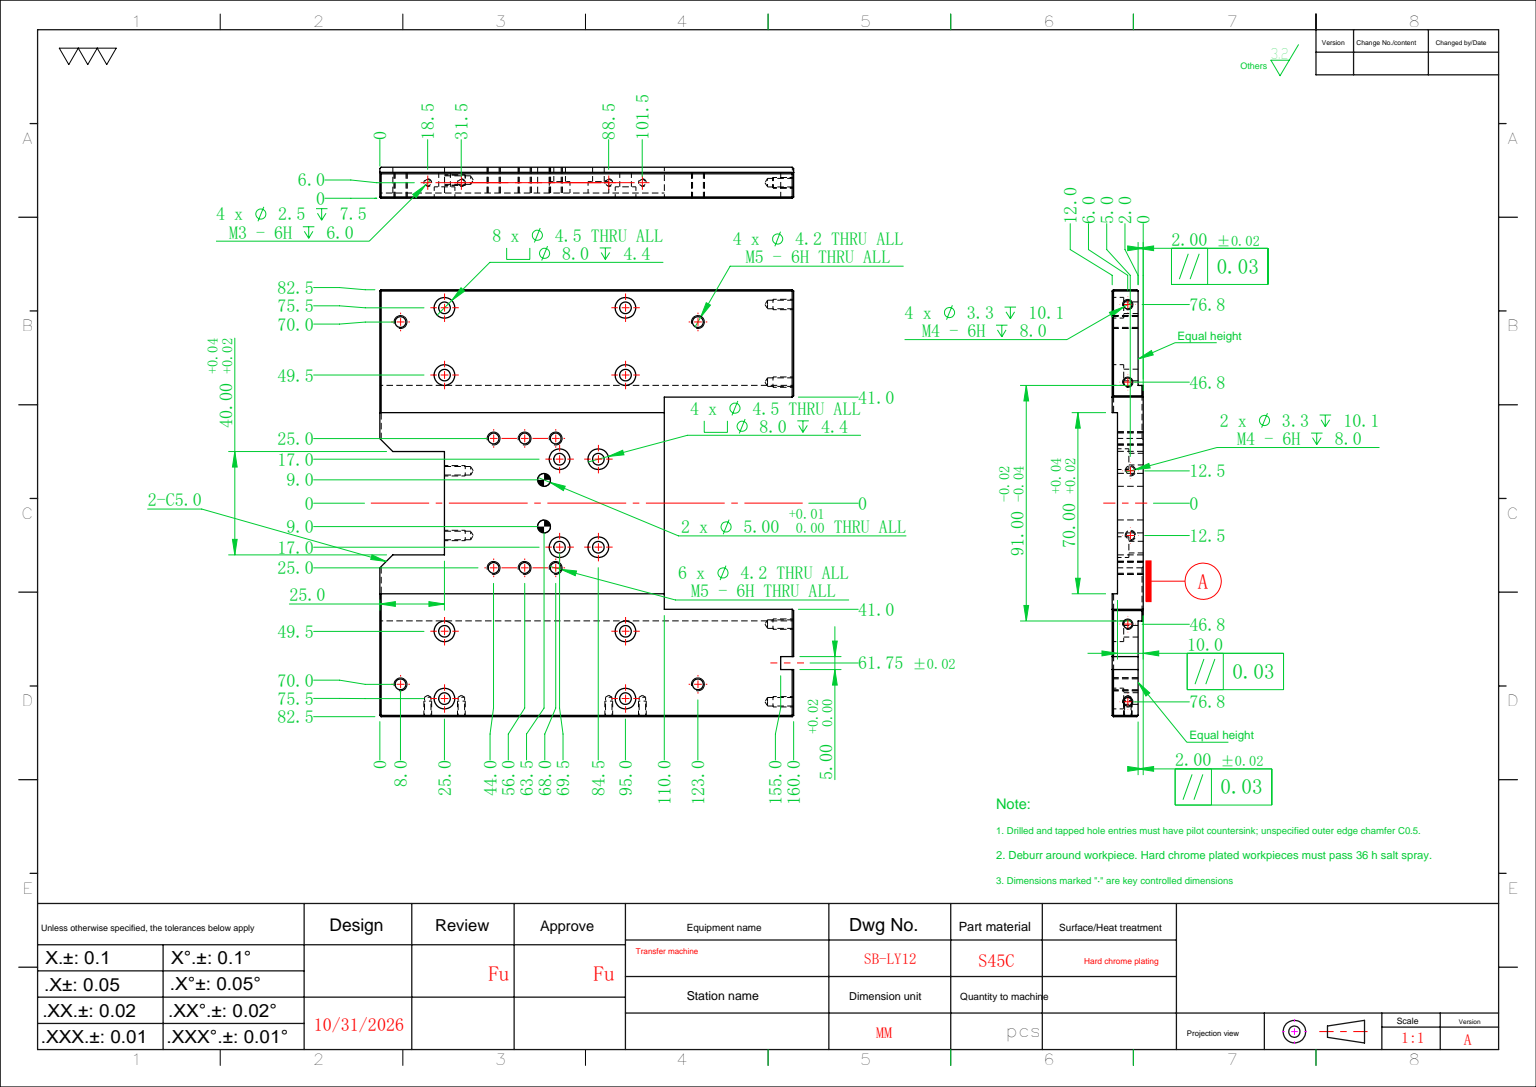
SolidWorks part; units mm, degrees
ref_plane "前视基准面" through (0, 0, 0) normal (0, 0, 1) x (1, 0, 0)
ref_plane "上视基准面" through (0, 0, 0) normal (0, 1, 0) x (1, 0, 0)
ref_plane "右视基准面" through (0, 0, 0) normal (1, 0, 0) x (0, 0, -1)
sketch "草图1" plane through (0, 0, 0) normal (0, 0, 1) x (1, 0, 0)
  line L1 (-80, -82.5) -> (80, -82.5)
  line L2 (-80, -82.5) -> (-80, 82.5)
  line L3 (-80, 82.5) -> (80, 82.5)
  line L4 (80, -82.5) -> (80, 82.5)
  line L5 (-80, -82.5) -> (80, 82.5) construction
  line L6 (-80, 82.5) -> (80, -82.5) construction
  point P0 (0, 0)
  dimension "D1" = 160
  dimension "D2" = 165
extrude "凸台-拉伸1" add sketch "草图1" along normal blind 12
sketch "草图2" plane through (0, 0, 0) normal (0, 0, -1) x (-1, 0, 0)
  line L0 (-80, -82.5) -> (-80, 82.5) construction
  line L1 (-80, -41) -> (-30, -41)
  line L2 (-80, -41) -> (-80, 41)
  line L3 (-80, 41) -> (-30, 41)
  line L4 (-30, -41) -> (-30, 41)
  line L5 (0, 0) -> (-82.6129, 0) construction
  dimension "D1" = 82
  dimension "D2" = 50
extrude "切除-拉伸1" cut sketch "草图2" against normal through all
sketch "草图3" plane through (-80, 0, 0) normal (-1, 0, 0) x (0, 0, 1)
  line L0 (12, 82.5) -> (12, -82.5) construction
  line L1 (12, 79.5) -> (10, 79.5)
  line L2 (12, 79.5) -> (12, 45.5)
  line L3 (12, 45.5) -> (10, 45.5)
  line L4 (10, 79.5) -> (10, 45.5)
  line L5 (0, 0) -> (47.3737, 0) construction
  line L6 (0, 82.5) -> (0, -82.5) construction
  line L7 (10, -79.5) -> (10, -45.5)
  line L8 (12, -45.5) -> (10, -45.5)
  line L9 (12, -79.5) -> (12, -45.5)
  line L10 (12, -79.5) -> (10, -79.5)
  line L11 (10, 62.5) -> (22.1068, 62.5) construction
  line L12 (10, -62.5) -> (25.4571, -62.5) construction
  dimension "D1" = 34
  dimension "D2" = 2
  dimension "D3" = 125
extrude "切除-拉伸2" cut sketch "草图3" against normal through all
hole_wizard "M4 六角凹头螺钉的柱形沉头孔2" positions "草图4" profile "草图5" counterbore size "M4" standard "ISO" end condition through all
sketch "草图4" plane through (0, 0, 0) normal (0, 0, -1) x (-1, 0, 0)
  line L0 (-80, 62.5) -> (-23.5435, 62.5) construction
  line L1 (-80, 79.5) -> (-80, 45.5) construction
  line L3 (0, 0) -> (127.4178, 0) construction
  line L5 (-80, -62.5) -> (-23.5435, -62.5) construction
  line L6 (-80, -45.5) -> (-80, -79.5) construction
  point P0 (-15, 49.5)
  point P2 (-15, 75.5)
  point P19 (-15, -75.5)
  point P20 (-15, -49.5)
  point P30 (55, -75.5)
  point P34 (55, -49.5)
  point P35 (55, 49.5)
  point P37 (55, 75.5)
  dimension "D1" = 26
  dimension "D3" = 65
  dimension "D5" = 70
sketch "草图5" plane through (15, 49.5, 0) normal (1, 0, 0) x (0, 1, 0)
  line L0 (0, 0) -> (0, 12)
  line L1 (0, 12) -> (2.25, 12)
  line L3 (2.25, 12) -> (2.25, 4.4)
  line L4 (2.25, 4.4) -> (4, 4.4)
  line L5 (4, 4.4) -> (4, 0)
  line L7 (4, 0) -> (0, 0)
  line L11 (0, -6.35) -> (0, 107.95) construction
  dimension "通孔孔直径" = 4.5
  dimension "通孔孔深度" = 12
  dimension "柱形沉头孔直径" = 8
  dimension "柱形沉头孔深度" = 4.4
sketch "草图6" plane through (0, 0, 0) normal (0, 0, -1) x (-1, 0, 0)
  line L0 (80, 82.5) -> (80, -82.5) construction
  line L1 (80, -35) -> (-30, -35)
  line L2 (80, -35) -> (80, 35)
  line L3 (80, 35) -> (-30, 35)
  line L4 (-30, -35) -> (-30, 35)
  line L5 (-30, -41) -> (-30, 41) construction
  line L8 (0, 0) -> (92.3084, 0) construction
  dimension "D1" = 70
extrude "切除-拉伸3" cut sketch "草图6" against normal blind 2
hole_wizard "M4 六角凹头螺钉的柱形沉头孔1" positions "草图7" profile "草图8" counterbore size "M4" standard "ISO" end condition through all
sketch "草图7" plane through (0, 0, 2) normal (0, 0, -1) x (-1, 0, 0)
  line L0 (0, 0) -> (106.2768, 0) construction
  line L1 (-30, -41) -> (-30, 41) construction
  point P0 (-4.5, -17)
  point P2 (-4.5, 17)
  point P4 (10.5, -17)
  point P6 (10.5, 17)
  dimension "D1" = 34
  dimension "D2" = 15
  dimension "D3" = 25.5
sketch "草图8" plane through (4.5, -17, 2) normal (1, 0, 0) x (0, 1, 0)
  line L0 (0, 0) -> (0, 10)
  line L1 (0, 10) -> (2.25, 10)
  line L3 (2.25, 10) -> (2.25, 4.4)
  line L4 (2.25, 4.4) -> (4, 4.4)
  line L5 (4, 4.4) -> (4, 0)
  line L7 (4, 0) -> (0, 0)
  line L11 (0, -6.35) -> (0, 107.95) construction
  dimension "通孔孔直径" = 4.5
  dimension "通孔孔深度" = 10
  dimension "柱形沉头孔直径" = 8
  dimension "柱形沉头孔深度" = 4.4
hole_wizard "大小mm 暗销孔2" positions "草图11" profile "草图12" hole size "Ø5.0" standard "ISO" end condition through all
sketch "草图11" plane through (0, 0, 2) normal (0, 0, -1) x (-1, 0, 0)
  line L0 (0, 0) -> (48.3077, 0) construction
  circle A0 centre (10.5, 17) radius 4 construction
  point P0 (16.5, -9)
  point P2 (16.5, 9)
  dimension "D1" = 18
  dimension "D2" = 6
sketch "草图12" plane through (-16.5, -9, 2) normal (1, 0, 0) x (0, 1, 0)
  line L0 (0, 0) -> (0, 10)
  line L1 (0, 10) -> (2.5, 10)
  line L2 (2.5, 10) -> (2.5, 0)
  line L5 (2.5, 0) -> (0, 0)
  line L11 (0, -6.35) -> (0, 107.95) construction
  dimension "通孔孔直径" = 5
  dimension "通孔孔深度" = 10
hole_wizard "M5 螺纹孔1" positions "草图13" profile "草图14" tap size "M5" standard "ISO" end condition through all
sketch "草图13" plane through (0, 0, 0) normal (0, 0, -1) x (-1, 0, 0)
  line L2 (0, 0) -> (134.1177, 0) construction
  line L3 (80, 82.5) -> (80, 35) construction
  point P0 (72, 70)
  point P3 (-43, 70)
  point P26 (-43, -70)
  point P27 (72, -70)
  dimension "D1" = 115
  dimension "D2" = 123
  dimension "D3" = 140
sketch "草图14" plane through (-72, 70, 0) normal (1, 0, 0) x (0, 1, 0)
  line L0 (0, 0) -> (0, 12)
  line L1 (0, 12) -> (2.1, 12)
  line L2 (2.1, 12) -> (2.1, 0)
  line L5 (2.1, 0) -> (0, 0)
  line L11 (0, -6.35) -> (0, 107.95) construction
  dimension "通孔螺纹孔钻头直径" = 4.2
  dimension "通孔螺纹孔钻头深度" = 12
cosmetic thread "孔螺蚊线1" parameters "D2"=5
cosmetic thread "孔螺蚊线2" parameters "D2"=5
cosmetic thread "孔螺蚊线3" parameters "D2"=5
cosmetic thread "孔螺蚊线4" parameters "D2"=5
hole_wizard "M4 螺纹孔1" positions "草图15" profile "草图16" tap size "M4" standard "ISO"
sketch "草图15" plane through (80, 0, 0) normal (1, 0, 0) x (0, 0, -1)
  line L0 (0, 61.75) -> (-19.2056, 61.75) construction
  line L1 (0, 41) -> (0, 82.5) construction
  line L3 (0, 0) -> (-26.7426, 0) construction
  point P0 (-6, 76.75)
  point P3 (-6, 46.75)
  point P21 (-6, -46.75)
  point P22 (-6, -76.75)
  dimension "D1" = 30
  dimension "D2" = 6
sketch "草图16" plane through (80, 76.75, 6) normal (0, 1, 0) x (0, 0, -1)
  line L0 (0, 0) -> (0, 11.0914)
  line L1 (0, 11.0914) -> (1.65, 10.1)
  line L2 (1.65, 10.1) -> (1.65, 0)
  line L5 (1.65, 0) -> (0, 0)
  line L10 (0, 11.0914) -> (-1.65, 10.1) construction
  line L11 (0, -6.35) -> (0, 107.95) construction
  dimension "螺纹孔钻头直径" = 3.3
  dimension "螺纹孔钻头深度" = 10.1
  dimension "导头角度" = 118
cosmetic thread "孔螺蚊线5" parameters "D1"=8, "D2"=4
cosmetic thread "孔螺蚊线6" parameters "D1"=8, "D2"=4
cosmetic thread "孔螺蚊线7" parameters "D1"=8, "D2"=4
cosmetic thread "孔螺蚊线8" parameters "D1"=8, "D2"=4
sketch "草图17" plane through (80, 0, 0) normal (1, 0, 0) x (0, 0, -1)
  line L0 (0, 41) -> (0, 82.5) construction
  line L1 (0, 59.25) -> (-10, 59.25)
  line L2 (0, 59.25) -> (0, 64.25)
  line L3 (0, 64.25) -> (-10, 64.25)
  line L4 (-10, 59.25) -> (-10, 64.25)
  line L5 (-10, 79.5) -> (-10, 45.5) construction
  line L6 (-6, 46.75) -> (-6, 76.75) construction
  line L7 (-6, 61.75) -> (6.0988, 61.75) construction
  dimension "D1" = 5
extrude "切除-拉伸4" cut sketch "草图17" against normal blind 5
hole_wizard "M5 螺纹孔2" positions "草图18" profile "草图19" tap size "M5" standard "ISO" end condition through all
sketch "草图18" plane through (0, 0, 2) normal (0, 0, -1) x (-1, 0, 0)
  line L0 (0, 0) -> (64.1152, 0) construction
  line L2 (80, 82.5) -> (80, 35) construction
  point P0 (12, 25)
  point P3 (12, -25)
  dimension "D1" = 50
  dimension "D2" = 68
sketch "草图19" plane through (-12, 25, 2) normal (1, 0, 0) x (0, 1, 0)
  line L0 (0, 0) -> (0, 10)
  line L1 (0, 10) -> (2.1, 10)
  line L2 (2.1, 10) -> (2.1, 0)
  line L5 (2.1, 0) -> (0, 0)
  line L11 (0, -6.35) -> (0, 107.95) construction
  dimension "通孔螺纹孔钻头直径" = 4.2
  dimension "通孔螺纹孔钻头深度" = 10
cosmetic thread "孔螺蚊线9" parameters "D2"=5
cosmetic thread "孔螺蚊线10" parameters "D2"=5
pattern_linear "阵列(线性)1" count 3 spacing 12 along (-1, 0, 0) of "M5 螺纹孔2"
cosmetic thread "孔螺蚊线11" parameters "D2"=5
cosmetic thread "孔螺蚊线12" parameters "D2"=5
cosmetic thread "孔螺蚊线13" parameters "D2"=5
cosmetic thread "孔螺蚊线14" parameters "D2"=5
sketch "草图20" plane through (0, 0, 0) normal (0, 0, -1) x (-1, 0, 0)
  line L0 (0, 0) -> (87.7204, 0) construction
  line L1 (80, -20) -> (55, -20)
  line L2 (80, -20) -> (80, 20)
  line L3 (80, 20) -> (55, 20)
  line L4 (55, -20) -> (55, 20)
  line L5 (80, -35) -> (80, 35) construction
  dimension "D1" = 40
  dimension "D2" = 25
extrude "切除-拉伸5" cut sketch "草图20" against normal through all
chamfer "倒角1" distance 5 angle 45 2 edges at (-80, 20, 7) (-80, -20, 7)
hole_wizard "M4 螺纹孔2" positions "草图21" profile "草图22" tap size "M4" standard "ISO"
sketch "草图21" plane through (-55, 0, 0) normal (-1, 0, 0) x (0, 0, 1)
  line L0 (0, 0) -> (12.6577, 0) construction
  line L2 (12, 45.5) -> (12, 25) construction
  point P0 (7, 12.5)
  point P3 (7, -12.5)
  dimension "D1" = 25
  dimension "D2" = 5
sketch "草图22" plane through (-55, 12.5, 7) normal (0, 1, 0) x (0, 0, 1)
  line L0 (0, 0) -> (0, 11.0914)
  line L1 (0, 11.0914) -> (1.65, 10.1)
  line L2 (1.65, 10.1) -> (1.65, 0)
  line L5 (1.65, 0) -> (0, 0)
  line L10 (0, 11.0914) -> (-1.65, 10.1) construction
  line L11 (0, -6.35) -> (0, 107.95) construction
  dimension "螺纹孔钻头直径" = 3.3
  dimension "螺纹孔钻头深度" = 10.1
  dimension "导头角度" = 118
cosmetic thread "孔螺蚊线15" parameters "D1"=8, "D2"=4
cosmetic thread "孔螺蚊线16" parameters "D1"=8, "D2"=4
hole_wizard "M3 螺纹孔1" positions "草图23" profile "草图24" tap size "M3" standard "ISO"
sketch "草图23" plane through (0, 82.5, 0) normal (0, 1, 0) x (1, 0, 0)
  line L0 (-80, -6) -> (-3.6554, -6) construction
  line L1 (-80, -12) -> (-80, 0) construction
  line L6 (-55, -2.2) -> (-55, 9.4635) construction
  point P0 (-61.5, -6)
  point P2 (-48.5, -6)
  dimension "D1" = 13
  dimension "D2" = 25
sketch "草图24" plane through (-61.5, 82.5, 6) normal (1, 0, 0) x (0, 0, 1)
  line L0 (0, 0) -> (0, 8.2511)
  line L1 (0, 8.2511) -> (1.25, 7.5)
  line L2 (1.25, 7.5) -> (1.25, 0)
  line L5 (1.25, 0) -> (0, 0)
  line L10 (0, 8.2511) -> (-1.25, 7.5) construction
  line L11 (0, -6.35) -> (0, 107.95) construction
  dimension "螺纹孔钻头直径" = 2.5
  dimension "螺纹孔钻头深度" = 7.5
  dimension "导头角度" = 118
cosmetic thread "孔螺蚊线17" parameters "D1"=6, "D2"=3
cosmetic thread "孔螺蚊线18" parameters "D1"=6, "D2"=3
pattern_linear "阵列(线性)2" count 2 spacing 70 along (1, 0, 0) of "M3 螺纹孔1"
cosmetic thread "孔螺蚊线19" parameters "D1"=6, "D2"=3
cosmetic thread "孔螺蚊线20" parameters "D1"=6, "D2"=3
sketch "草图25" plane through (80, 0, 0) normal (1, 0, 0) x (0, 0, -1)
  line L0 (0, 0) -> (-27.5225, 0) construction
  line L1 (-10, 79.5) -> (-12, 79.5)
  line L2 (-10, 79.5) -> (-10, 82.5)
  line L3 (-10, 82.5) -> (-12, 82.5)
  line L4 (-12, 79.5) -> (-12, 82.5)
  line L5 (-12, -79.5) -> (-12, -82.5)
  line L6 (-10, -82.5) -> (-12, -82.5)
  line L7 (-10, -79.5) -> (-10, -82.5)
  line L8 (-10, -79.5) -> (-12, -79.5)
extrude "切除-拉伸6" cut sketch "草图25" against normal through all
chamfer "倒角2" distance 0.5 angle 45 19 edges at (80, 43.25, 12) (80, 41, 6) (80, 50.125, 0) (-80, -35.25, 12) (-80, -82.5, 5) (80, -82.5, 5) (80, -43.25, 12) (80, -41, 6) (80, -61.75, 0) (0, -82.5, 0) (-80, -58.75, 0) (-80, 35.25, 12) (80, 82.5, 5) (-80, 82.5, 5) (80, 73.375, 0) (0, 82.5, 0) (-80, 58.75, 0) (0, -82.5, 10) (0, 82.5, 10)
